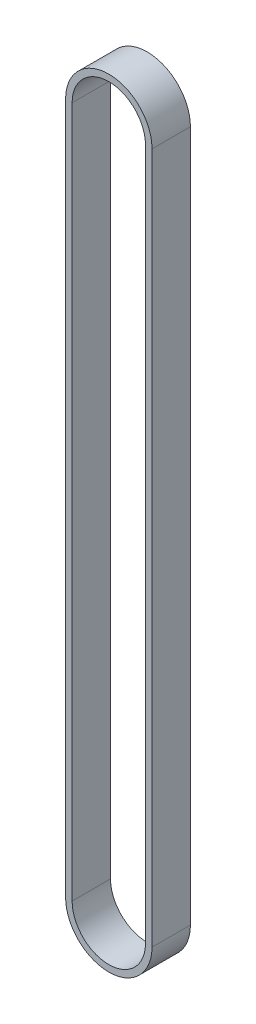
from build123d import *

# Parameters (mm, degrees)
BOSS_EXTRUDE1_DEPTH = 6


with BuildPart() as part:
    # Sketch1 → Boss-Extrude1 (new body)
    with BuildSketch(Plane.XY):
        with BuildLine():
            Line((-6.75, -54), (-6.75, 54))
            ThreePointArc((-6.75, 54), (0, 60.75), (6.75, 54))
            Line((6.75, 54), (6.75, -54))
            ThreePointArc((6.75, -54), (0, -60.75), (-6.75, -54))
        make_face()
        with BuildLine():
            Line((-5.73, -54), (-5.73, 54))
            ThreePointArc((-5.73, 54), (0, 59.73), (5.73, 54))
            Line((5.73, 54), (5.73, -54))
            ThreePointArc((5.73, -54), (0, -59.73), (-5.73, -54))
        make_face(mode=Mode.SUBTRACT)
    extrude(amount=BOSS_EXTRUDE1_DEPTH)


solid = part.part
